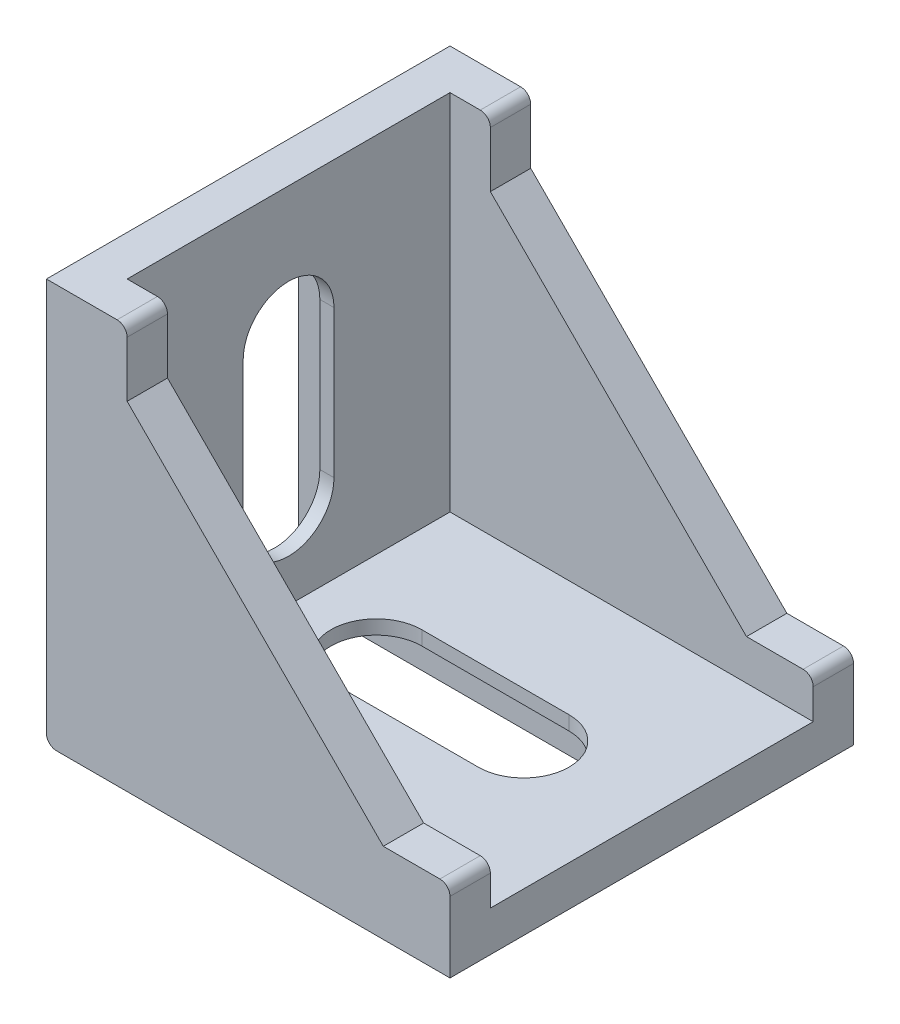
SolidWorks part; units mm, degrees
material "6063-T5 (GB)"
ref_plane "Front Plane" through (0, 0, 0) normal (0, 0, 1) x (1, 0, 0)
ref_plane "Top Plane" through (0, 0, 0) normal (0, 1, 0) x (1, 0, 0)
ref_plane "Right Plane" through (0, 0, 0) normal (1, 0, 0) x (0, 0, -1)
sketch "Sketch1" plane through (0, 0, 0) normal (0, 0, 1) x (1, 0, 0)
  line L1 (0, 0) -> (-40, 0)
  line L2 (0, 0) -> (0, 40)
  line L3 (0, 40) -> (-40, 40)
  line L4 (-40, 0) -> (-40, 40)
  dimension "D1" = 40
  dimension "D2" = 40
extrude "Boss-Extrude1" add sketch "Sketch1" along normal blind 40
sketch "Sketch2" plane through (0, 0, 40) normal (0, 0, 1) x (1, 0, 0)
  line L0 (-32, 40) -> (-32, 33.5)
  line L1 (0, 40) -> (-40, 40) construction
  line L2 (-32, 33.5) -> (-6.6106, 8)
  line L3 (-6.6106, 8) -> (0, 8)
  line L4 (0, 0) -> (0, 40) construction
  line L5 (-40, 0) -> (0, 0) construction
  line L6 (-40, 40) -> (-40, 0) construction
  line L7 (-32, 40) -> (-7.4956, 45.7139)
  line L8 (-7.4956, 45.7139) -> (17.0851, 36.2657)
  line L9 (17.0851, 36.2657) -> (0, 8)
  dimension "D1" = 8
  dimension "D2" = 6.5
  dimension "D3" = 8
extrude "Cut-Extrude1" cut sketch "Sketch2" against normal blind 40
sketch "Sketch3" plane through (0, 40, 0) normal (0, 1, 0) x (1, 0, 0)
  line L0 (0, 0) -> (0, -40) construction
  line L1 (-36, -4) -> (0, -4)
  line L2 (-36, -4) -> (-36, -36)
  line L3 (-36, -36) -> (0, -36)
  line L4 (0, -4) -> (0, -36)
  line L5 (-40, -40) -> (-40, 0) construction
  line L6 (-32, 0) -> (-6.6106, 0) construction
  line L7 (-32, -40) -> (-6.6106, -40) construction
  dimension "D1" = 4
  dimension "D2" = 4
  dimension "D3" = 4
extrude "Cut-Extrude2" cut sketch "Sketch3" against normal blind 36
sketch "Sketch4" plane through (0, 0, 0) normal (0, -1, 0) x (1, 0, 0)
  line L0 (-40, 40) -> (0, 40) construction
  line L1 (-37.8, 37.2) -> (-1.8, 37.2)
  line L2 (-37.8, 37.2) -> (-37.8, 31.2)
  line L3 (-37.8, 31.2) -> (-1.8, 31.2)
  line L4 (-1.8, 37.2) -> (-1.8, 31.2)
  line L5 (0, 40) -> (0, 0) construction
  line L7 (-40, 40) -> (-40, 0) construction
  line L8 (-35, 25) -> (-6, 25)
  line L9 (-35, 25) -> (-35, 15)
  line L10 (-35, 15) -> (-6, 15)
  line L11 (-6, 25) -> (-6, 15)
  line L12 (-40, 20) -> (8.9596, 20) construction
  line L13 (-37.8, 2.8) -> (-37.8, 8.8)
  line L14 (-1.8, 2.8) -> (-1.8, 8.8)
  line L15 (-37.8, 8.8) -> (-1.8, 8.8)
  line L16 (-37.8, 2.8) -> (-1.8, 2.8)
  point P8 (-6, 20)
  point P15 (-40, 20)
  dimension "D1" = 2.8
  dimension "D2" = 36
  dimension "D3" = 1.8
  dimension "D4" = 10
  dimension "D5" = 29
  dimension "D6" = 6
  dimension "D7" = 0
  dimension "D8" = 6
extrude "Cut-Extrude3" cut sketch "Sketch4" against normal blind 2.6
ref_plane "Plane1" through (0, 0, 20) normal (0, 0, -1) x (-1, 0, 0)
sketch "Sketch5" plane through (0, 0, 25) normal (0, 0, -1) x (-1, 0, 0)
  line L0 (0, 0) -> (0, 8) construction
  line L1 (6, 2.6) -> (35, 2.6) construction
  line L2 (6, 2.6) -> (6, 0) construction
  line L3 (35, 2.6) -> (35, 0) construction
  line L4 (31.8, 2.6) -> (35, 2.6)
  line L5 (37.8, 2.6) -> (1.8, 2.6) construction
  line L6 (35, 2.6) -> (38, 2.6)
  line L7 (38, 2.6) -> (38, -2.5)
  line L8 (38, -2.5) -> (31.8, 2.6)
  line L9 (40, 0) -> (0, 0) construction
  line L10 (6, 0) -> (6, -2.5)
  line L11 (6, -2.5) -> (2.7, 0)
  line L12 (37.8, 0) -> (1.8, 0) construction
  line L13 (2.7, 0) -> (6, 0)
  dimension "D1" = 25.8
  dimension "D2" = 38
  dimension "D3" = 2.5
  dimension "D4" = 2.5
  dimension "D5" = 3.3
extrude "Boss-Extrude2" add sketch "Sketch5" along normal blind 10
sketch "Sketch6" plane through (0, 0, 0) normal (0, -1, 0) x (1, 0, 0)
  line L0 (-2.7, 15) -> (-2.7, 25) construction
  line L1 (-38, 15) -> (-2.7, 15)
  line L2 (-38, 15) -> (-38, 16.25)
  line L3 (-38, 16.25) -> (-2.7, 16.25)
  line L4 (-2.7, 15) -> (-2.7, 16.25)
  line L5 (-38, 20) -> (-2.7, 20) construction
  line L6 (-38, 25) -> (-38, 15) construction
  line L7 (-22, 20) -> (22, 20) construction
  line L8 (-2.7, 25) -> (-2.7, 23.75)
  line L9 (-38, 23.75) -> (-2.7, 23.75)
  line L10 (-38, 25) -> (-38, 23.75)
  line L11 (-38, 25) -> (-2.7, 25)
  dimension "D1" = 7.5
extrude "Cut-Extrude4" cut sketch "Sketch6" along normal blind 10
sketch "Sketch7" plane through (0, 0, 8.8) normal (0, 0, -1) x (-1, 0, 0)
  line L0 (37.8, 0) -> (34.3, 2.6)
  line L1 (1.8, 2.6) -> (37.8, 2.6) construction
  line L2 (1.8, 2.6) -> (1.8, 0) construction
  line L3 (34.3, 2.6) -> (37.8, 2.6)
  line L4 (37.8, 2.6) -> (37.8, 0)
  dimension "D1" = 32.5
extrude "Boss-Extrude3" add sketch "Sketch7" along normal blind 6
pattern_linear "LPattern1" count 2 spacing 28.4 along (0, 0, 1) of "Boss-Extrude3"
sketch "Sketch9" plane through (0, 2.6, 0) normal (0, -1, 0) x (1, 0, 0)
  line L0 (-20, 40) -> (-20, 0) construction
  line L1 (-40, 40) -> (0, 40) construction
  line L2 (-40, 0) -> (0, 0) construction
  line L3 (-27.3, 20) -> (-12.7, 20) construction
  line L4 (-22, 20) -> (22, 20) construction
  line L5 (-27.3, 24.5) -> (-12.7, 24.5)
  line L6 (-27.3, 15.5) -> (-12.7, 15.5)
  line L7 (0, 40) -> (0, 0) construction
  arc A0 (-27.3, 24.5) -> (-27.3, 15.5) centre (-27.3, 20) ccw
  arc A1 (-12.7, 15.5) -> (-12.7, 24.5) centre (-12.7, 20) ccw
  point P10 (-20, 20)
  point P15 (-8.2, 20)
  dimension "D2" = 4.5
  dimension "D1" = 8.2
extrude "Cut-Extrude5" cut sketch "Sketch9" against normal blind 5
ref_plane "Plane2" through (-20, 20, 0) normal (-0.7071, 0.7071, 0) x (0.7071, 0.7071, 0)
mirror "Mirror1" about plane through (-20, 20, 0) normal (-0.7071, 0.7071, 0) of "Cut-Extrude5", "LPattern1", "Boss-Extrude3", "Cut-Extrude4", "Boss-Extrude2", "Cut-Extrude3"
fillet "Fillet1" radius 1 5 edges at (-32, 40, 2) (-32, 40, 38) (0, 8, 38) (0, 8, 2) (-40, 0, 20)
